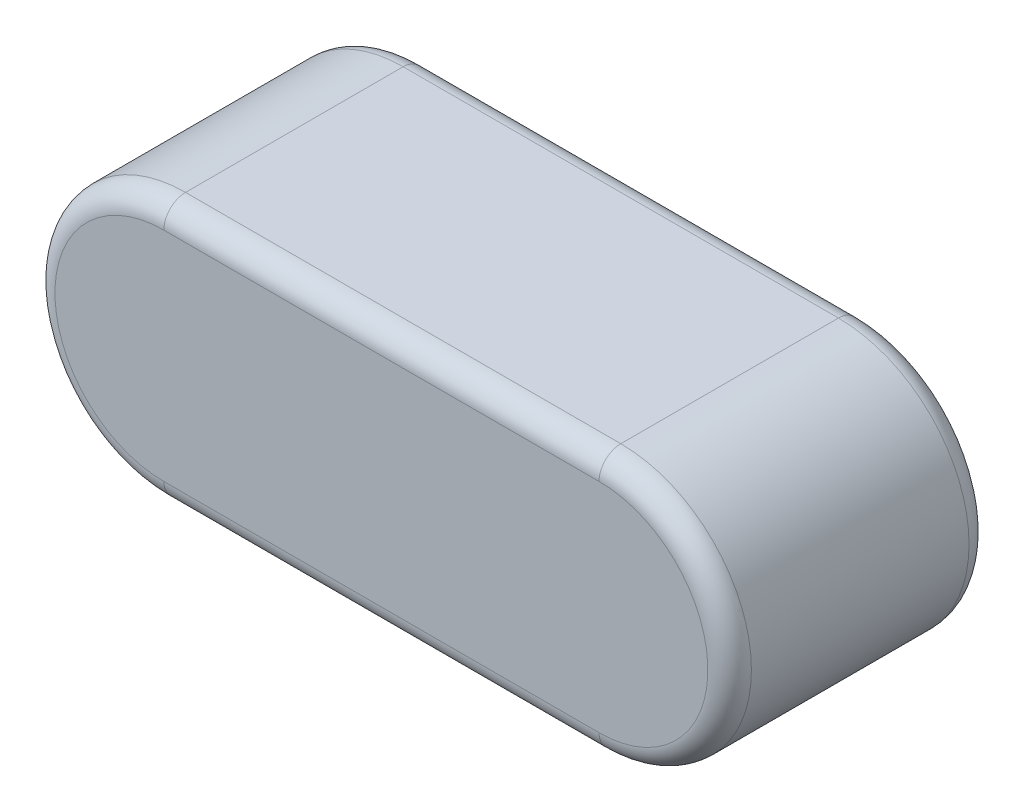
from build123d import *

# Parameters (mm, degrees)
BASE_EXTRUDE_DEPTH = 3
FILLET1_R          = 0.25


with BuildPart() as part:
    # Sketch1 → Base-Extrude (new body)
    with BuildSketch(Plane.XY):
        with BuildLine():
            Line((-2.5, 1.5), (2.5, 1.5))
            ThreePointArc((2.5, 1.5), (4, 0), (2.5, -1.5))
            Line((2.5, -1.5), (-2.5, -1.5))
            ThreePointArc((-2.5, -1.5), (-4, 0), (-2.5, 1.5))
        make_face()
    extrude(amount=BASE_EXTRUDE_DEPTH)

    # Fillet1
    fillet1_edges = [part.edges().sort_by_distance(p)[0] for p in [
        (4, 0, 3),
        (0, 1.5, 3),
        (-4, 0, 3),
        (0, 1.5, 0),
        (4, 0, 0),
        (0, -1.5, 0),
        (-4, 0, 0),
        (0, -1.5, 3),
    ]]
    fillet(fillet1_edges, radius=FILLET1_R)


solid = part.part
